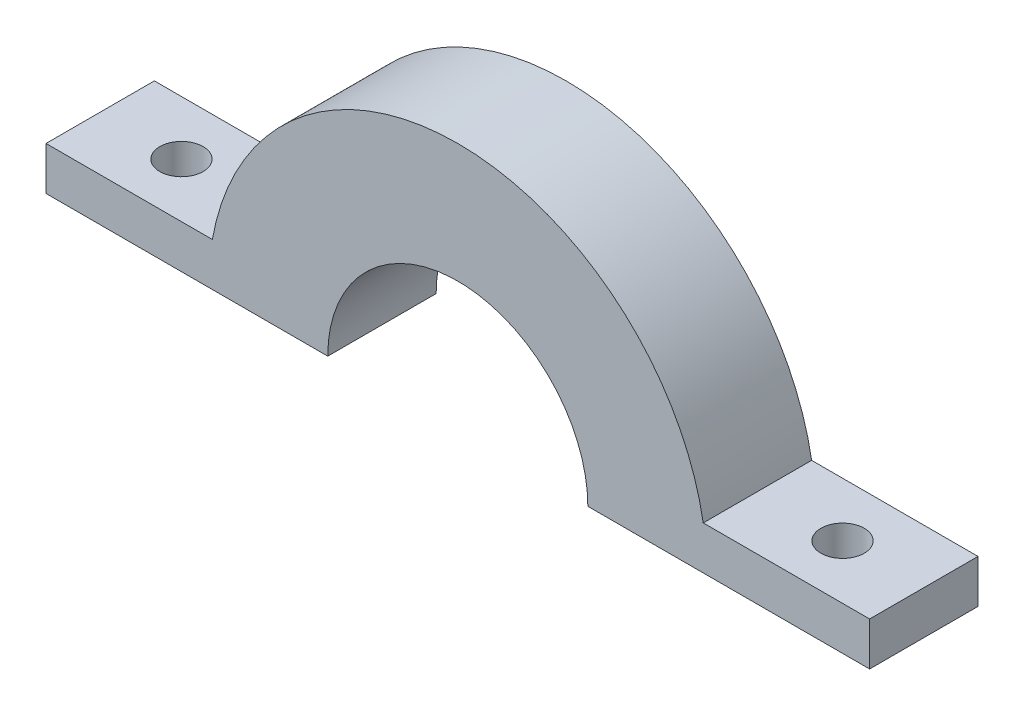
from build123d import *

# Parameters (mm, degrees)
BOSS_EXTRUDE1_DEPTH = 5
SKETCH3_R           = 1
CUT_EXTRUDE2_DEPTH  = 7
SKETCH4_R           = 6
CUT_EXTRUDE3_DEPTH  = 25.38777855


with BuildPart() as part:
    # Sketch2 → Boss-Extrude1 (new body)
    with BuildSketch(Plane.XY):
        with BuildLine():
            Line((9.583170828, 0), (17.083170828, 0))
            Line((17.083170828, 0), (17.083170828, 2))
            Line((17.083170828, 2), (9.407922481, 2))
            ThreePointArc((9.407922481, 2), (-1.916829172, 11.5), (-13.241580825, 2))
            Line((-13.241580825, 2), (-20.916829172, 2))
            Line((-20.916829172, 2), (-20.916829172, 0))
            Line((-20.916829172, 0), (-13.416829172, 0))
            Line((-13.416829172, 0), (-7.916829172, 0))
            Line((-7.916829172, 0), (4.083170828, 0))
            Line((4.083170828, 0), (9.583170828, 0))
        make_face()
    extrude(amount=BOSS_EXTRUDE1_DEPTH)

    # Sketch3 → Cut-Extrude2 (cut)
    with BuildSketch(Plane(origin=(0, 2, 0), x_dir=(1, 0, 0), z_dir=(0, 1, 0))):
        with Locations(Location((-17.166829172, -2.5, 0), (0, 0, 270))):
            Circle(SKETCH3_R)
        with Locations(Location((13.333170828, -2.5, 0), (0, 0, 270))):
            Circle(SKETCH3_R)
    extrude(amount=-CUT_EXTRUDE2_DEPTH, mode=Mode.SUBTRACT)

    # Sketch4 → Cut-Extrude3 (cut, through all)
    with BuildSketch(Plane.XY.offset(5)):
        with Locations((-1.916829172, 0)):
            Circle(SKETCH4_R)
    extrude(amount=-CUT_EXTRUDE3_DEPTH, mode=Mode.SUBTRACT)


solid = part.part
